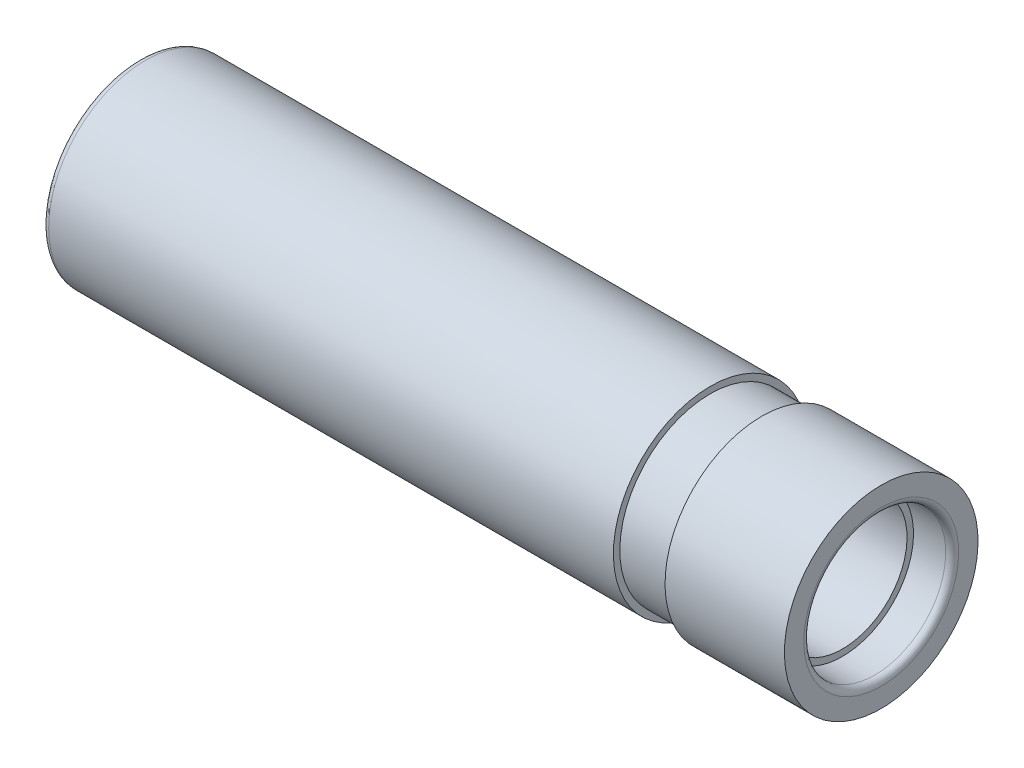
from build123d import *

# Parameters (mm, degrees)
FILLET1_R = 1


with BuildPart() as part:
    # Sketch1 → Revolve1 (revolve)
    with BuildSketch(Plane.XY):
        Polygon((-54.569644219, 7.757293726), (-54.569644219, 11.770249221), (33.930355781, 11.770249221), (33.930355781, 10.770249221), (41.930355781, 10.770249221), (41.930355781, 11.770249221), (60.430355781, 11.770249221), (60.430355781, 7.770249221), (54.430355781, 7.770249221), (54.430355781, 6.770249221), (-48.569644219, 6.770249221), (-48.569644219, 7.757293726), align=None)
    revolve(axis=Axis((54.430355781, -3.229750779, 0), (-1, 0, 0)))

    # Fillet1
    fillet1_edges = [part.edges().sort_by_distance(p)[0] for p in [
        (-54.569644219, -18.229750779, 0),
        (-54.569644219, -14.216795283, 0),
        (60.430355781, -14.229750779, 0),
    ]]
    fillet(fillet1_edges, radius=FILLET1_R)


solid = part.part
